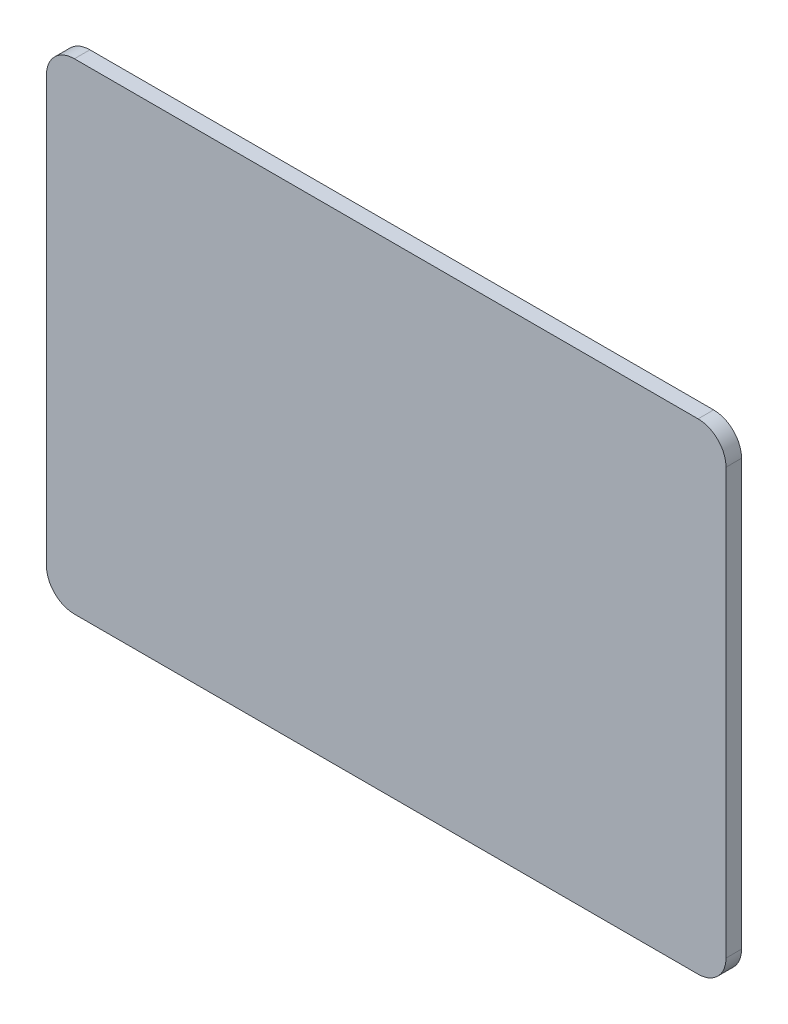
SolidWorks part; units mm, degrees
material "Plain Carbon Steel"
ref_plane "Front Plane" through (0, 0, 0) normal (0, 0, 1) x (1, 0, 0)
ref_plane "Top Plane" through (0, 0, 0) normal (0, 1, 0) x (1, 0, 0)
ref_plane "Right Plane" through (0, 0, 0) normal (1, 0, 0) x (0, 0, -1)
sketch "Sketch1" plane through (0, 0, 0) normal (0, 0, 1) x (1, 0, 0)
  line L1 (0, 0) -> (219, 0)
  line L2 (0, 0) -> (0, -155)
  line L3 (0, -155) -> (219, -155)
  line L4 (219, 0) -> (219, -155)
  dimension "D1" = 219
  dimension "D2" = 155
extrude "Boss-Extrude1" add sketch "Sketch1" along normal blind 5
fillet "Fillet1" radius 9 4 edges at (219, 0, 2.5) (219, -155, 2.5) (0, -155, 2.5) (0, 0, 2.5)
